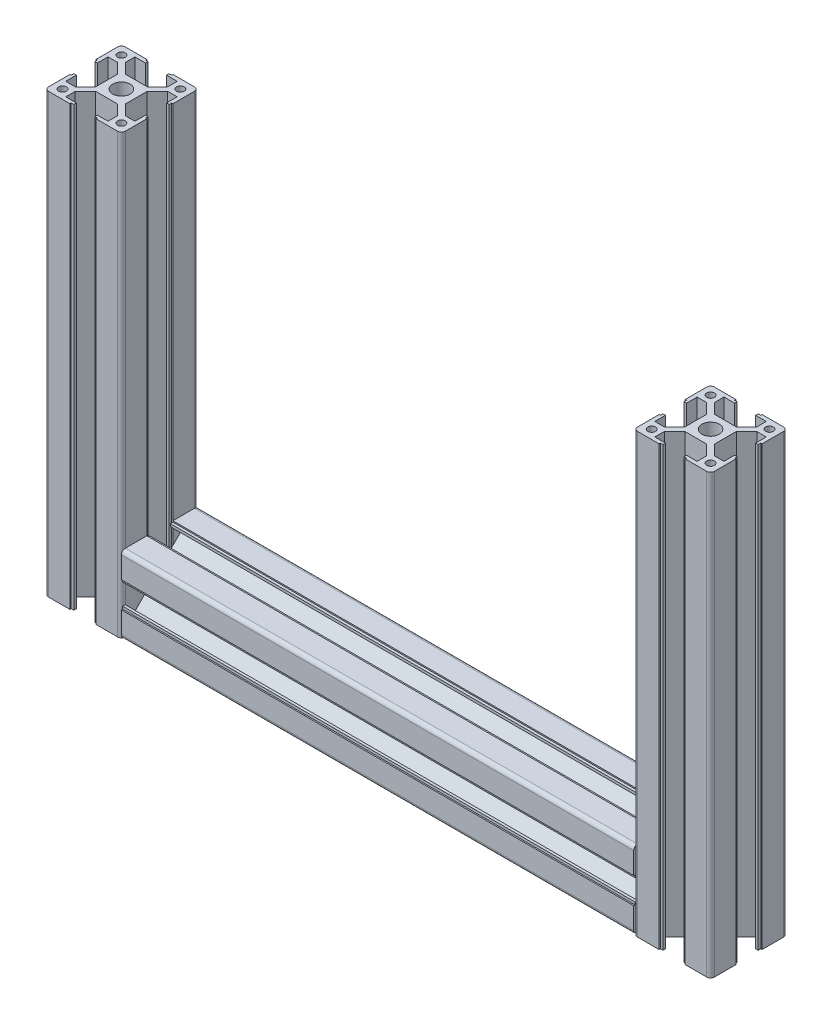
SolidWorks part; units mm, degrees
material "AL6061"
ref_plane "前视基准面" through (0, 0, 0) normal (0, 0, 1) x (1, 0, 0)
ref_plane "上视基准面" through (0, 0, 0) normal (0, 1, 0) x (1, 0, 0)
ref_plane "右视基准面" through (0, 0, 0) normal (1, 0, 0) x (0, 0, -1)
sketch "草图1" plane through (0, 0, 0) normal (0, 0, 1) x (1, 0, 0)
  line L1 (-115, 78) -> (115, 78)
  line L2 (-115, 78) -> (-115, -78)
  line L3 (-115, -78) -> (115, -78)
  line L4 (115, 78) -> (115, -78)
  line L5 (-115, 78) -> (115, -78) construction
  line L6 (-115, -78) -> (115, 78) construction
  point P0 (0, 0)
  dimension "D1" = 230
  dimension "D2" = 156
other "铝型材库 30X 30G X R1.5(1)"
ref_plane "基准面1" through (-115, 78, 0) normal (0, -1, 0) x (1, 0, 0)
sketch "Sketch11" plane through (-115, 78, 0) normal (0, -1, 0) x (1, 0, 0)
  line L0 (-5.1, 15) -> (-5.1, 14.5)
  line L1 (-5.1, 14.5) -> (-4.1, 14.5)
  line L2 (-4.1, 14.5) -> (-4.1, 13.5)
  line L3 (-4.1, 13.5) -> (-8.25, 13.5)
  line L4 (-13.5, -15) -> (-5.1, -15)
  line L5 (-15, -13.5) -> (-15, -5.1)
  line L6 (13.5, 15) -> (5.1, 15)
  line L7 (15, 13.5) -> (15, 5.1)
  line L8 (0, 14.8756) -> (0, 0) construction
  line L9 (0, 0) -> (14.1675, 0) construction
  line L10 (-8.25, 13.5) -> (-8.25, 9.8)
  line L11 (-8.25, 9.8) -> (-4.25, 5.8)
  line L12 (-4.25, 5.8) -> (4.25, 5.8)
  line L13 (8.25, 9.8) -> (4.25, 5.8)
  line L14 (8.25, 13.5) -> (8.25, 9.8)
  line L15 (4.1, 13.5) -> (8.25, 13.5)
  line L16 (4.1, 14.5) -> (4.1, 13.5)
  line L17 (5.1, 14.5) -> (4.1, 14.5)
  line L18 (5.1, 15) -> (5.1, 14.5)
  line L19 (-5.1, 15) -> (-13.5, 15)
  line L20 (15, 5.1) -> (14.5, 5.1)
  line L21 (14.5, 5.1) -> (14.5, 4.1)
  line L22 (14.5, 4.1) -> (13.5, 4.1)
  line L23 (13.5, 4.1) -> (13.5, 8.25)
  line L24 (13.5, 8.25) -> (9.8, 8.25)
  line L25 (9.8, 8.25) -> (5.8, 4.25)
  line L26 (5.8, 4.25) -> (5.8, -4.25)
  line L27 (9.8, -8.25) -> (5.8, -4.25)
  line L28 (13.5, -8.25) -> (9.8, -8.25)
  line L29 (13.5, -4.1) -> (13.5, -8.25)
  line L30 (14.5, -4.1) -> (13.5, -4.1)
  line L31 (14.5, -5.1) -> (14.5, -4.1)
  line L32 (15, -5.1) -> (14.5, -5.1)
  line L33 (5.1, -15) -> (5.1, -14.5)
  line L34 (5.1, -14.5) -> (4.1, -14.5)
  line L35 (4.1, -14.5) -> (4.1, -13.5)
  line L36 (4.1, -13.5) -> (8.25, -13.5)
  line L37 (8.25, -13.5) -> (8.25, -9.8)
  line L38 (8.25, -9.8) -> (4.25, -5.8)
  line L39 (4.25, -5.8) -> (-4.25, -5.8)
  line L40 (-8.25, -9.8) -> (-4.25, -5.8)
  line L41 (-8.25, -13.5) -> (-8.25, -9.8)
  line L42 (-4.1, -13.5) -> (-8.25, -13.5)
  line L43 (-4.1, -14.5) -> (-4.1, -13.5)
  line L44 (-5.1, -14.5) -> (-4.1, -14.5)
  line L45 (-5.1, -15) -> (-5.1, -14.5)
  line L46 (-15, -5.1) -> (-14.5, -5.1)
  line L47 (-14.5, -5.1) -> (-14.5, -4.1)
  line L48 (-14.5, -4.1) -> (-13.5, -4.1)
  line L49 (-13.5, -4.1) -> (-13.5, -8.25)
  line L50 (-13.5, -8.25) -> (-9.8, -8.25)
  line L51 (-9.8, -8.25) -> (-5.8, -4.25)
  line L52 (-5.8, -4.25) -> (-5.8, 4.25)
  line L53 (-9.8, 8.25) -> (-5.8, 4.25)
  line L54 (-13.5, 8.25) -> (-9.8, 8.25)
  line L55 (-13.5, 4.1) -> (-13.5, 8.25)
  line L56 (-14.5, 4.1) -> (-13.5, 4.1)
  line L57 (-14.5, 5.1) -> (-14.5, 4.1)
  line L58 (-15, 5.1) -> (-14.5, 5.1)
  line L59 (5.1, -15) -> (13.5, -15)
  line L60 (-15, 5.1) -> (-15, 13.5)
  line L61 (15, -5.1) -> (15, -13.5)
  circle A0 centre (0, 0) radius 3.4
  arc A1 (-15, 13.5) -> (-13.5, 15) centre (-13.5, 13.5) cw
  arc A2 (15, 13.5) -> (13.5, 15) centre (13.5, 13.5) ccw
  arc A3 (-13.5, -15) -> (-15, -13.5) centre (-13.5, -13.5) cw
  arc A4 (13.5, -15) -> (15, -13.5) centre (13.5, -13.5) ccw
  circle A5 centre (-11.5, 11.5) radius 1.5
  circle A6 centre (11.5, 11.5) radius 1.5
  circle A7 centre (-11.5, -11.5) radius 1.5
  circle A8 centre (11.5, -11.5) radius 1.5
  point P0 (-10, 0)
  point P1 (10, 0)
  point P2 (0, 10)
  point P3 (0, -10)
  point P4 (0, 0)
  point P5 (-15, -15)
  point P6 (15, -15)
  point P7 (15, 15)
  point P8 (-15, 15)
  point P36 (-15, 15)
  point P39 (15, 15)
  point P92 (0, 0)
  dimension "D1" = 16.5
  dimension "D2" = 30
  dimension "D3" = 8.2
  dimension "D4" = 10.2
  dimension "D5" = 9.2
  dimension "D6" = 6.8
  dimension "D7" = 1.5
  dimension "D8" = 45
  dimension "D12" = 3
  dimension "D13" = 23
  dimension "D14" = 23
  dimension "D9" = 0.5
  dimension "D10" = 1
  dimension "D11" = 8.5
